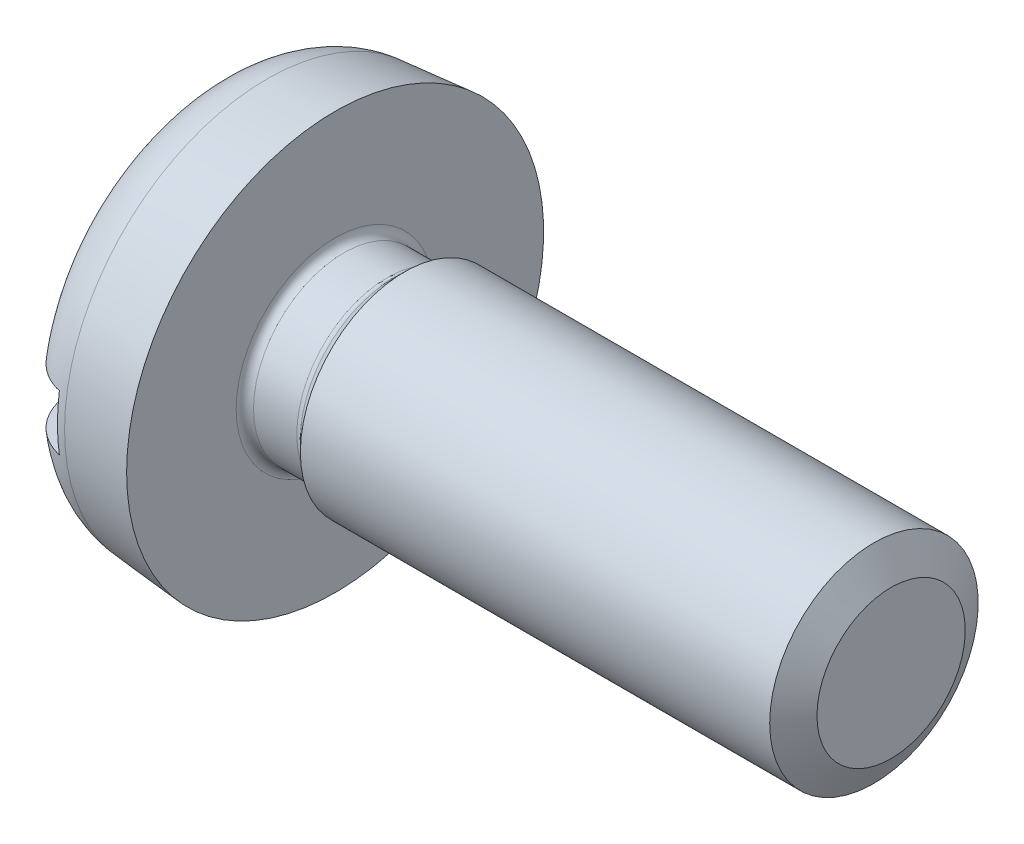
from build123d import *

# Parameters (mm, degrees)
FILLET1_R          = 0.25
FILLET2_R          = 1.8
SKETCH5_W          = 12
SKETCH5_H          = 1.6
CUT_EXTRUDE1_DEPTH = 1.4


with BuildPart() as part:
    # Sketch2 → Base-Revolve (revolve)
    with BuildSketch(Plane.XY, mode=Mode.PRIVATE) as base_revolve_sk:
        Polygon((0, 0), (19.6, 0), (19.6, 3), (5.6, 3), (5.198, 2.598), (3.6, 2.598), (3.6, 6), (0, 5.685040811), align=None)
    revolve(base_revolve_sk.sketch.rotate(Axis((-3.442001378, 0, 0), (1, 0, 0)), 90), axis=Axis((-3.442001378, 0, 0), (1, 0, 0)))

    # Fillet1
    fillet1_edges = [part.edges().sort_by_distance(p)[0] for p in [
        (3.6, 0, -2.598),
        (5.198, 0, -2.598),
    ]]
    fillet(fillet1_edges, radius=FILLET1_R)

    # Fillet2
    fillet2_edges = [part.edges().sort_by_distance(p)[0] for p in [
        (0, 0, -5.685040811),
    ]]
    fillet(fillet2_edges, radius=FILLET2_R)

    # Sketch5 → Cut-Extrude1 (cut)
    with BuildSketch(Plane(origin=(0, 0, 0), x_dir=(0, 0, -1), z_dir=(1, 0, 0))):
        Rectangle(SKETCH5_W, SKETCH5_H)
    extrude(amount=CUT_EXTRUDE1_DEPTH, mode=Mode.SUBTRACT)

    # Sketch3 → Cut-Revolve1 (revolve, cut)
    with BuildSketch(Plane.XY, mode=Mode.PRIVATE) as cut_revolve1_sk:
        Polygon((19.105416006, 3), (20.105416006, 3), (19.6, 2.134), align=None)
    revolve(cut_revolve1_sk.sketch.rotate(Axis((-0.122578865, 0, 0), (1, 0, 0)), 90), axis=Axis((-0.122578865, 0, 0), (1, 0, 0)), mode=Mode.SUBTRACT)


solid = part.part
